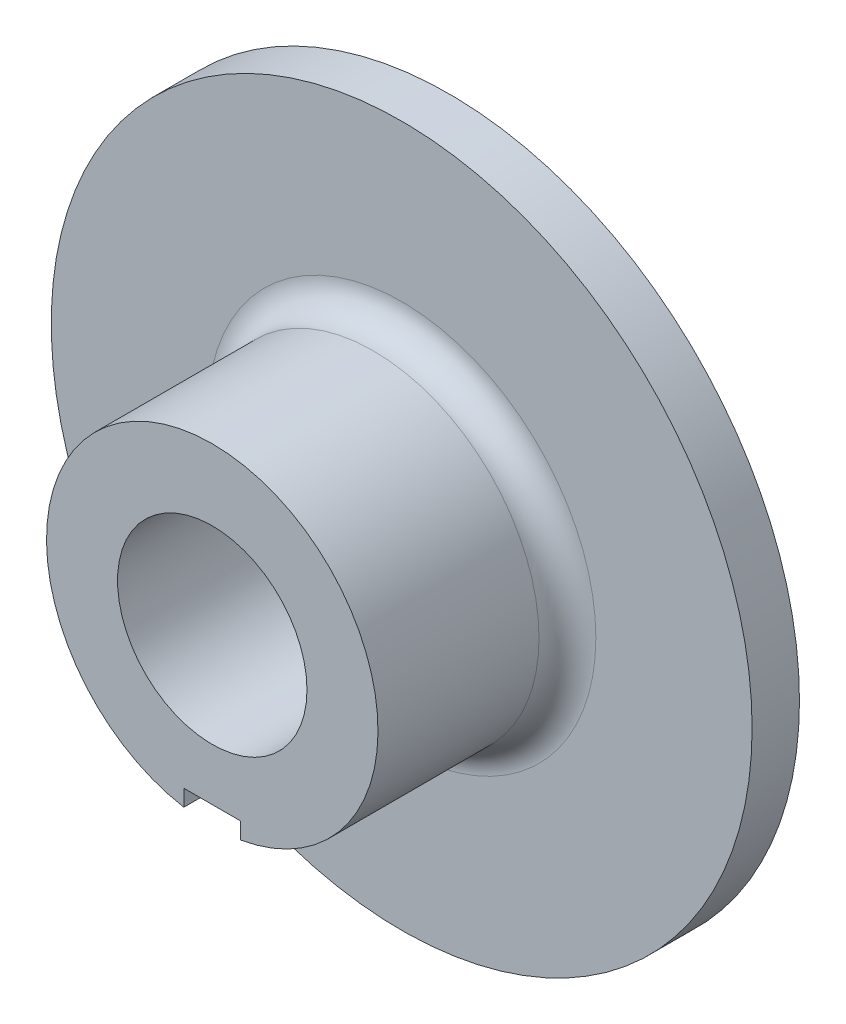
from build123d import *

# Parameters (mm, degrees)
SKETCH1_R           = 37
BOSS_EXTRUDE1_DEPTH = 5
SKETCH2_R           = 17.5
SKETCH2_R_2         = 10
BOSS_EXTRUDE2_DEPTH = 20
SKETCH3_R           = 10
CUT_EXTRUDE1_DEPTH  = 58.99137867
FILLET1_R           = 3
SKETCH4_W           = 6
SKETCH4_H           = 4
CUT_EXTRUDE2_DEPTH  = 17


with BuildPart() as part:
    # Sketch1 → Boss-Extrude1 (new body)
    with BuildSketch(Plane.XY):
        Circle(SKETCH1_R)
    extrude(amount=BOSS_EXTRUDE1_DEPTH)

    # Sketch2 → Boss-Extrude2 (add)
    with BuildSketch(Plane.XY.offset(5)):
        Circle(SKETCH2_R)
        Circle(SKETCH2_R_2, mode=Mode.SUBTRACT)
    extrude(amount=BOSS_EXTRUDE2_DEPTH)

    # Sketch3 → Cut-Extrude1 (cut, through all)
    with BuildSketch(Plane.XY.offset(25)):
        Circle(SKETCH3_R)
    extrude(amount=-CUT_EXTRUDE1_DEPTH, mode=Mode.SUBTRACT)

    # Fillet1
    fillet1_edges = [part.edges().sort_by_distance(p)[0] for p in [
        (-17.5, 0, 5),
    ]]
    fillet(fillet1_edges, radius=FILLET1_R)

    # Sketch4 → Cut-Extrude2 (cut)
    with BuildSketch(Plane.XY.offset(25)):
        with Locations((0, -17.5)):
            Rectangle(SKETCH4_W, SKETCH4_H)
    extrude(amount=-CUT_EXTRUDE2_DEPTH, mode=Mode.SUBTRACT)


solid = part.part
